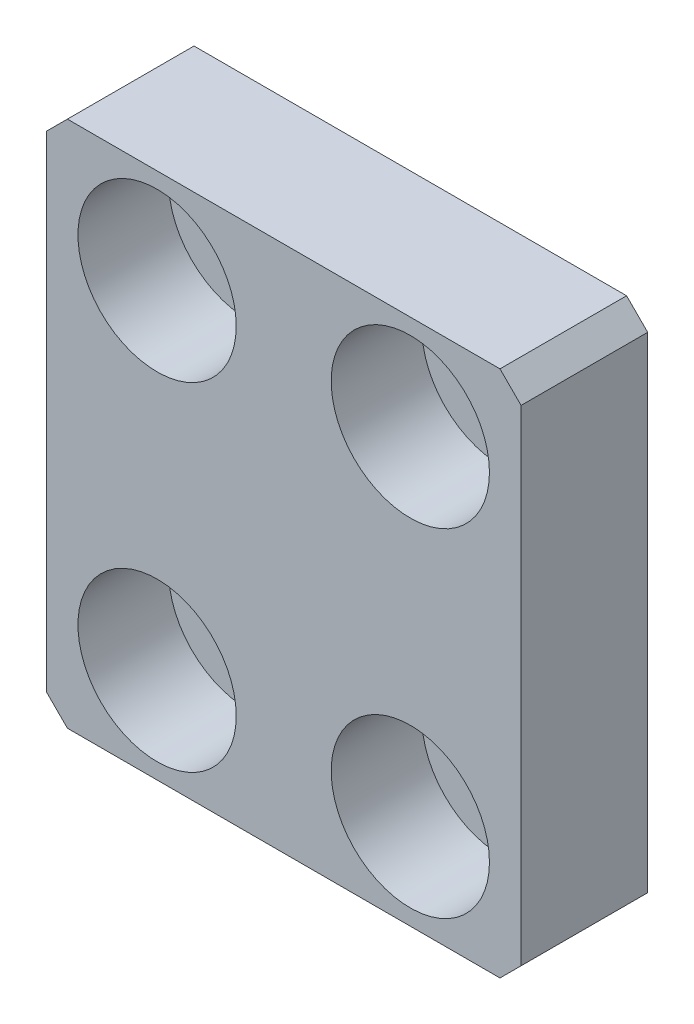
SolidWorks part; units mm, degrees
ref_plane "Front Plane" through (0, 0, 0) normal (0, 0, 1) x (1, 0, 0)
ref_plane "Top Plane" through (0, 0, 0) normal (0, 1, 0) x (1, 0, 0)
ref_plane "Right Plane" through (0, 0, 0) normal (1, 0, 0) x (0, 0, -1)
sketch "Sketch1" plane through (0, 0, 0) normal (0, 0, 1) x (1, 0, 0)
  line L1 (-22.5, 25) -> (22.5, 25)
  line L2 (-22.5, 25) -> (-22.5, -25)
  line L3 (-22.5, -25) -> (22.5, -25)
  line L4 (22.5, 25) -> (22.5, -25)
  line L5 (-22.5, 25) -> (22.5, -25) construction
  line L6 (-22.5, -25) -> (22.5, 25) construction
  point P0 (0, 0)
  dimension "D1" = 50
  dimension "D2" = 45
extrude "Boss-Extrude1" add sketch "Sketch1" along normal blind 12
hole_wizard "CBORE for M8 Hex Socket Head Cap Screw1" positions "Sketch4" profile "Sketch2" counterbore size "M8" standard "Iso" end condition through all
sketch "Sketch4" plane through (0, 0, 12) normal (0, 0, 1) x (1, 0, 0)
  line L0 (0, 0) -> (0, 45.3553) construction
  line L2 (0, 0) -> (-39.6325, 0) construction
  point P0 (-12, 16)
  point P17 (12, 16)
  point P18 (12, -16)
  point P19 (-12, -16)
  dimension "D1" = 12
  dimension "D2" = 16
sketch "Sketch2" plane through (-12, 16, 12) normal (1, 0, 0) x (0, -1, 0)
  line L0 (0, 0) -> (0, 12)
  line L1 (0, 12) -> (4.5, 12)
  line L3 (4.5, 12) -> (4.5, 8.6)
  line L4 (4.5, 8.6) -> (7.5, 8.6)
  line L5 (7.5, 8.6) -> (7.5, 0)
  line L7 (7.5, 0) -> (0, 0)
  line L11 (0, -6.35) -> (0, 107.95) construction
  dimension "通孔孔直径" = 9
  dimension "通孔孔深度" = 12
  dimension "柱形沉头孔直径" = 15
  dimension "柱形沉头孔深度" = 8.6
chamfer "Chamfer1" distance 2 angle 45 4 edges at (22.5, -25, 6) (-22.5, -25, 6) (22.5, 25, 6) (-22.5, 25, 6)
